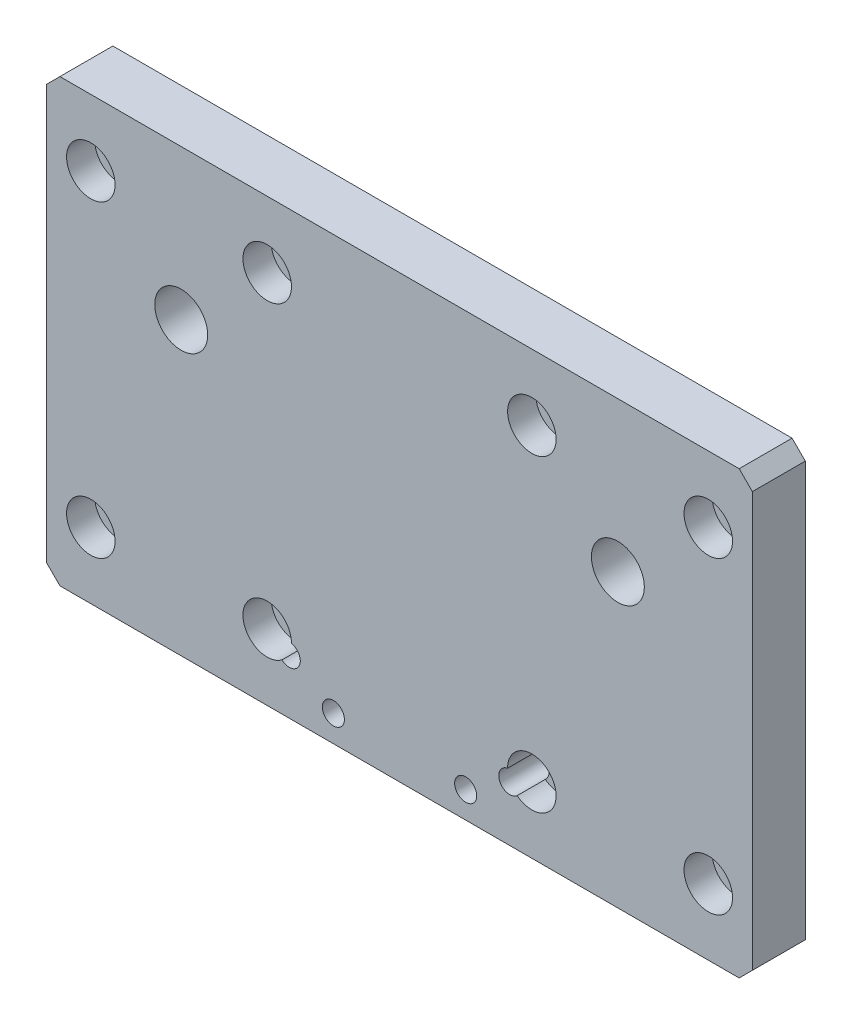
SolidWorks part; units mm, degrees
ref_plane "前视基准面" through (0, 0, 0) normal (0, 0, 1) x (1, 0, 0)
ref_plane "上视基准面" through (0, 0, 0) normal (0, 1, 0) x (1, 0, 0)
ref_plane "右视基准面" through (0, 0, 0) normal (1, 0, 0) x (0, 0, -1)
sketch "草图1" plane through (0, 0, 0) normal (0, 0, 1) x (1, 0, 0)
  line L1 (0, 0) -> (160, 0)
  line L2 (0, 0) -> (0, 100)
  line L3 (0, 100) -> (160, 100)
  line L4 (160, 0) -> (160, 100)
  dimension "D1" = 160
  dimension "D2" = 100
extrude "凸台-拉伸1" add sketch "草图1" along normal blind 12
hole_wizard "M14 螺纹孔1" positions "草图3" profile "草图2" tap size "M14" standard "GB" end condition through all
sketch "草图3" plane through (0, 0, 12) normal (0, 0, 1) x (1, 0, 0)
  line L0 (80, 0) -> (80, 89.6788) construction
  line L1 (0, 0) -> (160, 0) construction
  point P0 (30.5, 66)
  point P3 (129.5, 66)
  dimension "D1" = 99
  dimension "D2" = 66
sketch "草图2" plane through (30.5, 66, 12) normal (1, 0, 0) x (0, -1, 0)
  line L0 (0, 0) -> (0, 12)
  line L1 (0, 12) -> (6, 12)
  line L2 (6, 12) -> (6, 0)
  line L5 (6, 0) -> (0, 0)
  line L11 (0, -6.35) -> (0, 107.95) construction
  dimension "通孔螺纹孔钻头直径" = 12
  dimension "通孔螺纹孔钻头深度" = 12
cosmetic thread "孔螺蚊线1" parameters "D2"=14
cosmetic thread "孔螺蚊线2" parameters "D2"=14
hole_wizard "M6 六角凹头螺钉的柱形沉头孔1" positions "草图5" profile "草图4" counterbore size "M6" standard "ISO" end condition through all
sketch "草图5" plane through (0, 0, 12) normal (0, 0, 1) x (1, 0, 0)
  line L0 (80, 100) -> (80, -9.8806) construction
  line L1 (160, 100) -> (0, 100) construction
  line L3 (0, 50) -> (63.747, 50) construction
  line L4 (0, 100) -> (0, 0) construction
  point P0 (10, 15)
  point P3 (50, 15)
  point P6 (50, 85)
  point P9 (10, 85)
  point P12 (110, 15)
  point P15 (150, 15)
  point P18 (150, 85)
  point P21 (110, 85)
  dimension "D1" = 100
  dimension "D2" = 40
  dimension "D3" = 70
sketch "草图4" plane through (10, 15, 12) normal (1, 0, 0) x (0, -1, 0)
  line L0 (0, 0) -> (0, 12)
  line L1 (0, 12) -> (3.2, 12)
  line L3 (3.2, 12) -> (3.2, 6.4)
  line L4 (3.2, 6.4) -> (5.5, 6.4)
  line L5 (5.5, 6.4) -> (5.5, 0)
  line L7 (5.5, 0) -> (0, 0)
  line L11 (0, -6.35) -> (0, 107.95) construction
  dimension "通孔孔直径" = 6.4
  dimension "通孔孔深度" = 12
  dimension "柱形沉头孔直径" = 11
  dimension "柱形沉头孔深度" = 6.4
chamfer "倒角1" distance 3 angle 45 4 edges at (160, 0, 6) (160, 100, 6) (0, 0, 6) (0, 100, 6)
hole_wizard "M6 螺纹孔1" positions "草图7" profile "草图6" tap size "M6" standard "GB" end condition through all
sketch "草图7" plane through (0, 0, 0) normal (0, 0, -1) x (-1, 0, 0)
  point P0 (-65, 6)
  point P3 (-95, 6)
sketch "草图6" plane through (65, 6, 0) normal (1, 0, 0) x (0, 1, 0)
  line L0 (0, 0) -> (0, 12)
  line L1 (0, 12) -> (2.5, 12)
  line L2 (2.5, 12) -> (2.5, 0)
  line L5 (2.5, 0) -> (0, 0)
  line L11 (0, -6.35) -> (0, 107.95) construction
  dimension "通孔螺纹孔钻头直径" = 5
  dimension "通孔螺纹孔钻头深度" = 12
cosmetic thread "孔螺蚊线3" parameters "D2"=6
cosmetic thread "孔螺蚊线4" parameters "D2"=6
hole_wizard "M6 螺纹孔2" positions "草图9" profile "草图8" tap size "M6" standard "GB"
sketch "草图9" plane through (0, 0, 12) normal (0, 0, 1) x (1, 0, 0)
  point P0 (55, 12.5)
  point P3 (105, 12.5)
sketch "草图8" plane through (55, 12.5, 12) normal (1, 0, 0) x (0, -1, 0)
  line L0 (0, 0) -> (0, 16.5022)
  line L1 (0, 16.5022) -> (2.5, 15)
  line L2 (2.5, 15) -> (2.5, 0)
  line L5 (2.5, 0) -> (0, 0)
  line L10 (0, 16.5022) -> (-2.5, 15) construction
  line L11 (0, -6.35) -> (0, 107.95) construction
  dimension "螺纹孔钻头直径" = 5
  dimension "螺纹孔钻头深度" = 15
  dimension "导头角度" = 118
cosmetic thread "孔螺蚊线6" parameters "D1"=12, "D2"=6
cosmetic thread "孔螺蚊线7" parameters "D1"=12, "D2"=6
